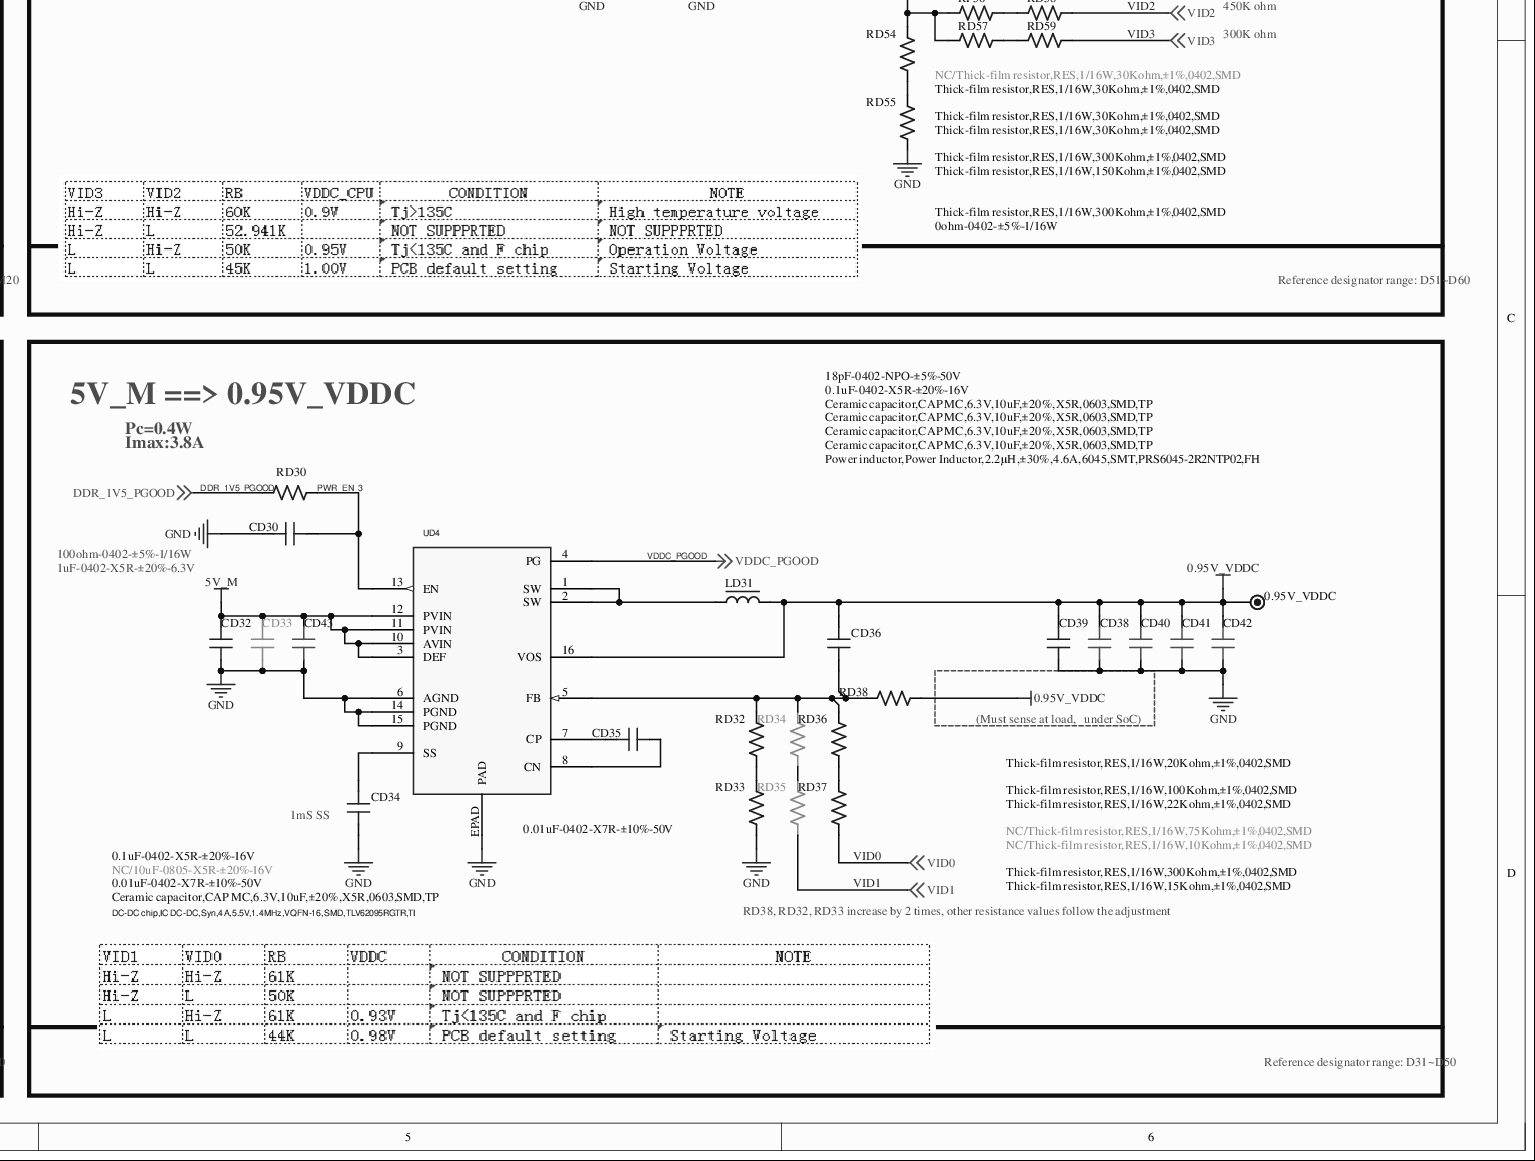
[diagram p0: MISC86290-6.SchDoc, bottom right]
# Altium project MISC86290.PrjPcb (part 5 of 13)

## Sheet MISC86290-6.SchDoc (continued)

### Parts
0.95V_VDDC  TEST  [TP]  (value not drawn)
1V5_DDR  TEST  [TP]  (value not drawn)
3V3_M  TEST  [TP]  (value not drawn)
3V3_STB  TEST  [TP]  (value not drawn)
3V3_Tun  TEST  [TP]  (value not drawn)
5V_M  TEST  [TP]  (value not drawn)
C58  NC/Ceramic capacitor,CAP MC,16V,0.1uF,±20%,X5R,0402,SMD,TP  [C0402]
CD1  NC/10uF-1206-X5R-±10%-16V  [C1206]
CD2  NC/1uF-0402-X5R-±20%-16V  [C0402]
CD3  10uF-0805-X5R-±20%-16V  [C0805]
CD4  NC/0.1uF-0402-X7R-±10%-16V  [C0402]
CD5  0.1uF-0402-X5R-±20%-16V  [C0402]
CD6  NC/8pF-0402-NPO-±5%-50V  [C0402]
CD7  NC/0.1uF-0402-X5R-±20%-16V  [C0402]
CD8  NC/Ceramic capacitor,CAP MC,6.3V,10uF,±20%,X5R,0603,SMD,TP  [C0603]
CD9  NC/Ceramic capacitor,CAP MC,6.3V,10uF,±20%,X5R,0603,SMD,TP  [C0603]
CD10  Ceramic capacitor,CAP MC,6.3V,10uF,±20%,X5R,0603,SMD,TP  [C0603]
CD11  10uF-0805-X5R-±20%-16V  [C0805]
CD12  NC/0.1uF-0402-X5R-±20%-16V  [C0402]
CD13  NC/10uF-1206-X5R-±10%-16V  [C1206]
CD14  0.1uF-0402-X5R-±20%-16V  [C0402]
CD15  NC/8pF-0402-NPO-±5%-50V  [C0402]
CD16  NC/0.1uF-0402-X5R-±20%-16V  [C0402]
CD17  Ceramic capacitor,CAP MC,6.3V,10uF,±20%,X5R,0603,SMD,TP  [C0603]
CD18  Ceramic capacitor,CAP MC,6.3V,10uF,±20%,X5R,0603,SMD,TP  [C0603]
CD19  Ceramic capacitor,CAP MC,6.3V,10uF,±20%,X5R,0603,SMD,TP  [C0603]
CD21  Ceramic capacitor,CAP MC,6.3V,10uF,±20%,X5R,0603,SMD,TP  [C0603]
CD22  0.1uF-0402-X7R-±10%-16V  [C0402]
CD23  Ceramic capacitor,CAP MC,50V,18pF,±5%,NPO,0402,SMD,TP  [C0402]
CD25  Ceramic capacitor,CAP MC,6.3V,10uF,±20%,X5R,0603,SMD,TP  [C0603]
CD26  Ceramic capacitor,CAP MC,6.3V,10uF,±20%,X5R,0603,SMD,TP  [C0603]
CD27  Ceramic capacitor,CAP MC,6.3V,22uF,±20%,X5R,0603,SMD,TP  [C0603]
CD29  0.1uF-0402-X7R-±10%-16V  [C0402]
CD30  1uF-0402-X5R-±20%-6.3V  [C0402]
CD32  0.1uF-0402-X5R-±20%-16V  [C0402]
CD33  NC/10uF-0805-X5R-±20%-16V  [C0805]
CD34  0.01uF-0402-X7R-±10%-50V  [C0402]
CD35  0.01uF-0402-X7R-±10%-50V  [C0402]
CD36  18pF-0402-NPO-±5%-50V  [C0402]
CD38  Ceramic capacitor,CAP MC,6.3V,10uF,±20%,X5R,0603,SMD,TP  [C0603]
CD39  0.1uF-0402-X5R-±20%-16V  [C0402]
CD40  Ceramic capacitor,CAP MC,6.3V,10uF,±20%,X5R,0603,SMD,TP  [C0603]
CD41  Ceramic capacitor,CAP MC,6.3V,10uF,±20%,X5R,0603,SMD,TP  [C0603]
CD42  Ceramic capacitor,CAP MC,6.3V,10uF,±20%,X5R,0603,SMD,TP  [C0603]
CD43  Ceramic capacitor,CAP MC,6.3V,10uF,±20%,X5R,0603,SMD,TP  [C0603]
CD51  Ceramic capacitor,CAP MC,6.3V,10uF,±20%,X5R,0603,SMD,TP  [C0603]
CD52  1uF-0402-X5R-±20%-6.3V  [C0402]
CD53  Ceramic capacitor,CAP MC,50V,18pF,±5%,NPO,0402,SMD,TP  [C0402]
CD54  Ceramic capacitor,CAP MC,6.3V,10uF,±20%,X5R,0603,SMD,TP  [C0603]
CD55  Ceramic capacitor,CAP MC,6.3V,10uF,±20%,X5R,0603,SMD,TP  [C0603]
CD56  Ceramic capacitor,CAP MC,6.3V,22uF,±20%,X5R,0603,SMD,TP  [C0603]
CG1  NC/1uF-0402-X5R-±20%-6.3V  [C0402]
CG11  NC/1uF-0402-X5R-±20%-6.3V  [C0402]
CG30  NC/1uF-0402-X5R-±20%-6.3V  [C0402]
CL1  0.1uF-0402-X5R-±20%-16V  [C0402]
CL2  Ceramic capacitor,CAP MC,6.3V,10uF,±20%,X5R,0603,SMD,TP  [C0603]
CL3  NC/0.1uF-0402-X5R-±20%-16V  [C0402]
CL13  Ceramic capacitor,CAP MC,6.3V,10uF,±20%,X5R,0603,SMD,TP  [C0603]
CL25  NC/0.1uF-0402-X5R-±20%-16V  [C0402]
CL55  0.1uF-0402-X5R-±20%-16V  [C0402]
CM1  1uF-0402-X5R-±20%-6.3V  [C0402]
CM2  0.022uF-0402-X7R-±10%-16V  [C0402]
CM3  22uF-0603-X5R-±20%-6.3V  [C0603]
CM4  0.022uF-0402-X7R-±10%-16V  [C0402]
CM15  NC/0.1uF-0402-X5R-±20%-16V  [C0402]
CM16  0.022uF-0402-X7R-±10%-16V  [C0402]
CM17  NC/10uF-0805-X5R-±20%-16V  [C0805]
CM18  NC/10uF-0805-X5R-±20%-16V  [C0805]
CNP2  Connector socket,connect jack,2×8Pin,D2.0,D,SNAP,L=2.6mm,DIP,CNJST  [SIP2*8/2.0D-5]
CP1  10uF-0805-X5R-±20%-16V  [C0805]
CP2  NC/0.1uF-0402-X5R-±20%-16V  [C0402]
DG1  NC/SFI0402-240E-2R5PP-LF  [DIODE-S0402]
DG11  NC/SFI0402-240E-2R5PP-LF  [DIODE-S0402]
DM11  NC/Switching diode,DIO SW S,150mA,75V,SOD-323,SMD,1N4148WS,BLUE ROCKET  [DIODE-S-12]
ED1  Aluminium electrolytic capacitor,CAP AL,10V,470uF,±20%,PKZH,P,2.5mm,6.3×11,DIP,TP,Koshin  [EC(6.3*11)-V-2.5]
EP1  Aluminium electrolytic capacitor,CAP AL,16V,220uF,±20%,LD,KF,P,2.5mm,6.3×11,DIP,TP,CapXon  [EC(6.3*11)-V-2.5]
LD1  NC/Power inductor,Power Inductor,4.7uH,±20%,3.3A,DR6.0×4.5,SMD,SWPA6045S4R7MT,Sunlord  [L(6.0*4.5)-S]
LD2  Power inductor,Power Inductor,4.7uH,±20%,2.8A,0.32×1P,DR5.8×4.5,SMD,PIO54-4R7MTP02,FH  [L(5.8*4.5)-S]
LD3  NC/Power inductor,Power Inductor,4.7uH,±20%,3.8A,DR6.0×4.5,SMD,MPIT6045-4R7M-LF,Microgate  [L(6.0*4.5)-S]
LD4  Power inductor,Power Inductor,4.7uH,±20%,3.3A,DR6.0×4.5,SMD,PRS6045-4R7MTP02,FH  [L(6.0*4.5)-S]
LD21  Power inductor,Power Inductor,2.2uH,±20%,2A,0.28×1P,DR4.5×3.2,SMD,PIO43-2R2MTP02,FH  [L(4.5*3.5)-S]
LD31  Power inductor,Power Inductor,2.2μH,±30%,4.6A,6045,SMT,PRS6045-2R2NTP02,FH  [L(6.0*4.5)-S]
LD51  Power inductor,Power Inductor,2.2uH,±20%,2A,0.28×1P,DR4.5×3.2,SMD,PIO43-2R2MTP02,FH  [L(4.5*3.5)-S]
MOD_1V2  TEST  [TP]
QG1  NC/General-purpose transistor,Dynatron,NPN,0.2A,40V,60-300,SOT-23,KMBT3904,KEXIN  [SOT-23]
QG2  NC/General-purpose transistor,Dynatron,NPN,0.2A,40V,60-300,SOT-23,KMBT3904,KEXIN  [SOT-23]
QG11  NC/General-purpose transistor,Dynatron,NPN,0.2A,40V,60-300,SOT-23,KMBT3904,KEXIN  [SOT-23]
QG12  NC/General-purpose transistor,Dynatron,NPN,0.2A,40V,60-300,SOT-23,KMBT3904,KEXIN  [SOT-23]
QG30  NC/General-purpose transistor,Dynatron,NPN,0.2A,40V,60-300,SOT-23,KMBT3904,KEXIN  [SOT-23]
QG31  NC/General-purpose transistor,Dynatron,NPN,0.2A,40V,60-300,SOT-23,KMBT3904,KEXIN  [SOT-23]
QM1  MOSFET,PMOS,-4.2A,-30V,0.052ohm@ID=-4.2A@VGS=-10V,SOT23-3,AO3401,BLUE ROCKET  [SOT-23-1]
QM2  MOSFET,PMOS,-5.7A,-30V,0.07ohm@ID=-4.4A@VGS=-4.5V,SOP-8,KO4459,KEXIN  [SO-8]
QM4  General-purpose transistor,Dynatron,NPN,0.2A,40V,60-300,SOT-23,KMBT3904,KEXIN  [SOT-23]
QM11  General-purpose transistor,Dynatron,NPN,0.2A,40V,60-300,SOT-23,KMBT3904,KEXIN  [SOT-23]
RD1  100ohm-0402-±5%-1/16W  [R0402]
RD2  NC/1Mohm-0402-±5%-1/16W  [R0402]
RD3  0ohm-0402-±5%-1/16W  [R0402]
RD4  0ohm-0402-±5%-1/16W  [R0402]
RD5  Thick-film resistor,RES,1/16W,59Kohm,±1%,0402,SMD  [R0402]
RD6  Thick-film resistor,RES,1/16W,10Kohm,±1%,0402,SMD  [R0402]
RD11  10Kohm-0402-±5%-1/16W  [R0402]
RD12  10Kohm-0402-±5%-1/16W  [R0402]
RD13  0ohm-0402-±5%-1/16W  [R0402]
RD14  0ohm-0402-±5%-1/16W  [R0402]
RD15  33Kohm-0402-±1%-1/16W  [R0402]
RD16  10Kohm-0402-±1%-1/16W  [R0402]
RD21  100Kohm-0402-±5%-1/16W  [R0402]
RD22  Thick-film resistor,RES,1/16W,15Kohm,±1%,0402,SMD  [R0402]
RD23  Thick-film resistor,RES,1/16W,10Kohm,±1%,0402,SMD  [R0402]
RD24  10Kohm-0402-±5%-1/16W  [R0402]
RD30  100ohm-0402-±5%-1/16W  [R0402]
RD32  Thick-film resistor,RES,1/16W,100Kohm,±1%,0402,SMD  [R0402]
RD33  Thick-film resistor,RES,1/16W,22Kohm,±1%,0402,SMD  [R0402]
RD34  NC/Thick-film resistor,RES,1/16W,75Kohm,±1%,0402,SMD  [R0402]
RD35  NC/Thick-film resistor,RES,1/16W,10Kohm,±1%,0402,SMD  [R0402]
RD36  Thick-film resistor,RES,1/16W,300Kohm,±1%,0402,SMD  [R0402]
RD37  Thick-film resistor,RES,1/16W,15Kohm,±1%,0402,SMD  [R0402]
RD38  Thick-film resistor,RES,1/16W,20Kohm,±1%,0402,SMD  [R0402]
RD51  NC/0ohm-0402-±5%-1/16W  [R0402]
RD52  10Kohm-0402-±5%-1/16W  [R0402]
RD53  NC/Thick-film resistor,RES,1/16W,30Kohm,±1%,0402,SMD  [R0402]
RD54  Thick-film resistor,RES,1/16W,30Kohm,±1%,0402,SMD  [R0402]
RD55  Thick-film resistor,RES,1/16W,30Kohm,±1%,0402,SMD  [R0402]
RD57  Thick-film resistor,RES,1/16W,300Kohm,±1%,0402,SMD  [R0402]
RD58  Thick-film resistor,RES,1/16W,150Kohm,±1%,0402,SMD  [R0402]
RD59  0ohm-0402-±5%-1/16W  [R0402]
RD60  Thick-film resistor,RES,1/16W,30Kohm,±1%,0402,SMD  [R0402]
RF56  Thick-film resistor,RES,1/16W,300Kohm,±1%,0402,SMD  [R0402]
RG1  NC/1Kohm-0402-±5%-1/16W  [R0402]
RG2  NC/4K7ohm-0402-±5%-1/16W  [R0402]
RG3  NC/33ohm-0402-±5%-1/16W  [R0402]
RG4  4K7ohm-0402-±5%-1/16W  [R0402]
RG5  100ohm-0402-±5%-1/16W  [R0402]
RG6  NC/10Kohm-0402-±5%-1/16W  [R0402]
RG7  NC/1Kohm-0402-±5%-1/16W  [R0402]
RG8  NC/10Kohm-0402-±5%-1/16W  [R0402]
RG11  NC/10Kohm-0402-±5%-1/16W  [R0402]
RG12  NC/1Kohm-0402-±5%-1/16W  [R0402]
RG13  NC/33ohm-0402-±5%-1/16W  [R0402]
RG14  4K7ohm-0402-±5%-1/16W  [R0402]
RG15  100ohm-0402-±5%-1/16W  [R0402]
RG16  NC/10Kohm-0402-±5%-1/16W  [R0402]
RG17  NC/1Kohm-0402-±5%-1/16W  [R0402]
RG18  NC/10Kohm-0402-±5%-1/16W  [R0402]
RG30  NC/4K7ohm-0402-±5%-1/16W  [R0402]
RG31  4K7ohm-0402-±5%-1/16W  [R0402]
RG32  NC/100ohm-0402-±5%-1/16W  [R0402]
RG33  100ohm-0402-±5%-1/16W  [R0402]
RG34  NC/10Kohm-0402-±5%-1/16W  [R0402]
RG35  0ohm-0402-±5%-1/16W  [R0402]
RG36  NC/10Kohm-0402-±5%-1/16W  [R0402]
RG37  NC/1Kohm-0402-±5%-1/16W  [R0402]
RG38  NC/1Kohm-0402-±5%-1/16W  [R0402]
RG39  NC/33ohm-0402-±5%-1/16W  [R0402]
RG40  NC/2K2ohm-0402-±5%-1/16W  [R0402]
RM1  15Kohm-0402-±1%-1/16W  [R0402]
RM2  4K7ohm-0402-±5%-1/16W  [R0402]
RM3  47Kohm-0402-±5%-1/16W  [R0402]
RM4  1Kohm-0402-±5%-1/16W  [R0402]
RM11  4K7ohm-0402-±5%-1/16W  [R0402]
RM12  10Kohm-0402-±5%-1/16W  [R0402]
RM13  4K7ohm-0402-±5%-1/16W  [R0402]
RM14  47Kohm-0402-±5%-1/16W  [R0402]
RM15  NC/4K7ohm-0402-±5%-1/16W  [R0402]
RP1  4K7ohm-0402-±5%-1/16W  [R0402]
RP5  NC/4K7ohm-0402-±5%-1/16W  [R0402]
RP8  100ohm-0402-±5%-1/16W  [R0402]
UD1  DC-DC chip,IC DCDC,Syn,4A,17V,500KHz,SOT23-6,SMD,TPS564201,TI  [SOP6/0.95]
UD2  DC-DC chip,IC DCDC,Syn,3A,17V,580KHz,TSOT23-6,SMD,TPS563201DDCR,TI  [SOP6/0.95]
UD3  DC-DC chip,IC DCDC,Syn,2A,5.5V,1.5MHz,SOT23-6,SMD,TLV62569PDDCR,TI  [SOT-23-6]
UD4  DC-DC chip,IC DC-DC,Syn,4A,5.5V,1.4MHz,VQFN-16,SMD,TLV62095RGTR,TI  [QFN16/0.5-4]
UD5  DC-DC chip,IC DCDC,Syn,2A,5.5V,1.5MHz,SOT23-6,SMD,TLV62569PDDCR,TI  [SOT-23-6]
UL1  LC1117CLTR33  [SOT-223]
UL2  LDO chip,IC LDO,1A,1.2V,15V,SOT-223,SMD,LC1117CLTR12,Leadchip  [SOT-223]
VCC_Panel  TEST  [TP]  (value not drawn)

### Blocks framed on the sheet
Power interface: CNP2 CP1 CP2 EP1 RP1 RP5 RP8
12V=>5V_M: 5V_M CD1-CD10 ED1 LD1 LD4 RD1-RD6 UD1
12V=>3V3_STB: 3V3_STB CD11-CD19 CD29 LD2 LD3 RD11-RD16 UD2
3V3_STB =>1V5_DDR: 1V5_DDR C58 CD21-CD23 CD25-CD27 LD21 RD21-RD24 UD3
5V_M ==> 0.95V_VDDCPU: CD51-CD56 LD51 RD51-RD55 RD57-RD60 RF56 UD5
PANEL VCC: CM15-CM18 DM11 QM2 QM11 RM11-RM15 VCC_Panel
3V3_STB=>3V3_M: 3V3_M CM1-CM4 QM1 QM4 RM1-RM4
BL_ON: CG1 DG1 QG1 QG2 RG1-RG8
5V_M ==> 0.95V_VDDC: 0.95V_VDDC CD30 CD32-CD36 CD38-CD43 LD31 RD30 RD32-RD38 UD4
PWM/ADJ: CG11 DG11 QG11 QG12 RG11-RG18
ADIM: CG30 QG30 QG31 RG30-RG40

### Nets
0.95V_VDDC: 0.95V_VDDC.1 CD36.2 CD38.2 CD39.2 CD40.2 CD41.2 CD42.2 LD31.2 RD38.2 UD4.16(VOS)
0.95V_VDDCPU: CD53.2 CD54.2 CD55.2 CD56.2 LD51.2 RD53.2 RD60.1
1V5_DDR: 1V5_DDR.1 C58.2 CD23.2 CD25.2 CD26.2 CD27.2 LD21.2 RD22.2
3V3_M: 3V3_M.1 CL55.2 CM2.2 CM3.2 QM1.D RD24.2 RG6.2 RG16.2 RP5.2 UL2.3(VI)
3V3_STB: 3V3_STB.1 CD15.2 CD16.2 CD17.2 CD18.2 CD19.2 CD21.2 CM4.2 LD2.1 LD3.2 QM1.S RD15.1 RD21.2 RG7.2 RG17.2 RG30.2 RG38.2 RM2.1 RP1.2 UD3.4(VIN)
3V3_Tun: 3V3_Tun.1 CL2.2 CL3.1 UL1.2(VO) UL1.4(VO)
5V_M: 5V_M.1 CD7.2 CD8.2 CD9.2 CD10.2 CD32.2 CD33.1 CD43.2 CD51.2 CL1.1 ED1.1 LD1.2 LD4.2 RD5.1 RD52.2 RG1.2 RG12.2 RG37.2 UD4.3(DEF) UD4.10(AVIN) UD4.11(PVIN) UD4.12(PVIN) UD5.4(VIN) UL1.3(VI)
12V: CD1.2 CD2.2 CD3.1 CD11.1 CD12.2 CD13.2 CM15.2 CNP2.5 CNP2.6 CNP2.7 CNP2.8 CP1.2 CP2.2 EP1.1 QM2.1(S) QM2.2(S) QM2.3(S) RD11.1 RM13.1 UD1.3(IN) UD2.3(IN)
AMP_VCC: CNP2.1 CNP2.2
GND: C58.1 CD1.1 CD2.1 CD3.2 CD4.2 CD6.1 CD7.1 CD8.1 CD9.1 CD10.1 CD11.2 CD12.1 CD13.1 CD16.1 CD17.1 CD18.1 CD19.1 CD21.1 CD22.2 CD25.1 CD26.1 CD27.1 CD29.2 CD30.1 CD32.1 CD33.2 CD34.1 CD38.1 CD39.1 CD40.1 CD41.1 CD42.1 CD43.1 CD51.1 CD52.2 CD54.1 CD55.1 CD56.1 CG1.1 CG11.1 CG30.1 CL1.2 CL2.1 CL3.2 CL13.1 CL25.1 CL55.1 CM1.1 CM3.1 CM17.2 CM18.2 CNP2.3 CNP2.4 CNP2.9 CNP2.10 CNP2.11 CNP2.12 CP1.1 CP2.1 DG1.A DG11.A ED1.2 EP1.2 QG1.E QG2.E QG11.E QG12.E QG30.E QG31.E QM4.E QM11.E RD2.1 RD6.1 RD12.1 RD16.1 RD23.1 RD33.1 RD55.1 RG4.1 RG14.1 RG31.1 RG40.1 RM12.1 RM15.2 UD1.1(GND) UD2.1(GND) UD3.2(GND) UD4.6(AGND) UD4.14(PGND) UD4.15(PGND) UD4.EPAD(PAD) UD5.2(GND) UL1.1(ADJ) UL2.1(ADJ)
MOD_1V2: CL13.2 CL25.2 MOD_1V2.1 UL2.2(VO) UL2.4(VO)
VCC_Panel: CM16.2 CM17.1 CM18.1 QM2.5(D) QM2.6(D) QM2.7(D) QM2.8(D) RM15.1 VCC_Panel.1
BL_ADIM: CG30.2 CNP2.14 RG35.1 RG39.2 RG40.2
BL_ON: CG1.2 CNP2.15 RG3.1 RG4.2 RG5.1
DDR_1V5_PGOOD: RD24.1 RD30.1 RD51.2 UD3.5(PG) ; off-sheet DDR_1V5_PGOOD
PS_ON: CNP2.13 RP5.1 RP8.1
PWM/ADJ: CG11.2 CNP2.16 RG13.2 RG14.2 RG15.1
PWR_EN_3: CD30.2 RD30.2 UD4.13(EN)
SOC_BL_ADIM: RG33.1 ; off-sheet SOC_BL_ADIM
SOC_BL_ON: DG1.K RG2.2 RG5.2 RG6.1 ; off-sheet SOC_BL_ON
SOC_BL_PDIM: DG11.K RG11.2 RG15.2 RG16.1 ; off-sheet SOC_BL_PDIM
SOC_BOOSTER: RG32.1 ; off-sheet SOC_BOOSTER
SOC_PANEL_ON: RM11.1 RM12.2 ; off-sheet SOC_PANEL_ON
SOC_PS_ON: RD1.1 RM1.1 RP1.1 RP8.2 ; off-sheet SOC_PS_ON
VDDC_PGOOD: UD4.4(PG) ; off-sheet VDDC_PGOOD
VDDCPU_PGOOD: UD5.5(PG) ; off-sheet VDDCPU_PGOOD
VID0: RD37.1 ; off-sheet VID0
VID1: RD35.1 ; off-sheet VID1
VID2: RD58.1 ; off-sheet VID2
VID3: RD59.1 ; off-sheet VID3
NetCD4_1: CD4.1 RD1.2 RD2.2 UD1.5(EN)
NetCD5_1: CD5.1 RD3.2
NetCD5_2: CD5.2 LD1.1 LD4.1 UD1.2(SW)
NetCD6_2: CD6.2 RD4.1 UD1.4(FB)
NetCD14_1: CD14.1 LD2.2 LD3.1 UD2.2(SW)
NetCD14_2: CD14.2 RD13.2
NetCD15_1: CD15.1 RD14.2 RD15.2 RD16.2
NetCD22_1: CD22.1 RD21.1 UD3.1(EN)
NetCD23_1: CD23.1 RD22.1 RD23.2 UD3.6(FB)
NetCD29_1: CD29.1 RD11.2 RD12.2 UD2.5(EN)
NetCD34_2: CD34.2 UD4.9(SS)
NetCD35_1: CD35.1 UD4.8(CN)
NetCD35_2: CD35.2 UD4.7(CP)
NetCD36_1: CD36.1 RD32.1 RD34.1 RD36.1 RD38.1 UD4.5(FB)
NetCD52_1: CD52.1 RD51.1 RD52.1 UD5.1(EN)
NetCD53_1: CD53.1 RD53.1 RD54.2 RD57.2 RD60.2 RF56.2 UD5.6(FB)
NetCM1_2: CM1.2 QM4.B RM1.2
NetCM2_1: CM2.1 RM4.2
NetCM4_1: CM4.1 QM1.G RM3.2 RM4.1
NetCM15_1: CM15.1 CM16.1 DM11.K QM2.4(G) RM14.2
NetDM11_A: DM11.A QM11.C RM13.2 RM14.1
NetLD21_1: LD21.1 UD3.3(SW)
NetLD31_1: LD31.1 UD4.1(SW) UD4.2(SW)
NetLD51_1: LD51.1 UD5.3(SW)
NetQG1_B: QG1.B RG8.1
NetQG1_C: QG1.C RG1.1 RG3.2
NetQG2_B: QG2.B RG2.1
NetQG2_C: QG2.C RG7.1 RG8.2
NetQG11_B: QG11.B RG18.1
NetQG11_C: QG11.C RG12.1 RG13.1
NetQG12_B: QG12.B RG11.1
NetQG12_C: QG12.C RG17.1 RG18.2
NetQG30_B: QG30.B RG34.1
NetQG30_C: QG30.C RG36.2 RG38.1
NetQG31_B: QG31.B RG36.1
NetQG31_C: QG31.C RG37.1 RG39.1
NetQM4_C: QM4.C RM2.2 RM3.1
NetQM11_B: QM11.B RM11.2
NetRD3_1: RD3.1 UD1.6(BS)
NetRD4_2: RD4.2 RD5.2 RD6.2
NetRD13_1: RD13.1 UD2.6(BS)
NetRD14_1: RD14.1 UD2.4(FB)
NetRD32_2: RD32.2 RD33.2
NetRD34_2: RD34.2 RD35.2
NetRD36_2: RD36.2 RD37.2
NetRD54_1: RD54.1 RD55.2
NetRD57_1: RD57.1 RD59.2
NetRD58_2: RD58.2 RF56.1
NetRG30_1: RG30.1 RG31.2 RG32.2 RG33.2 RG34.2 RG35.2

### Notes on the sheet
- Imax:3.6A
- Pc=0.44W
- Pc=0.88W
- Imax:2.4A
- STR
- Imax:1A
- Pc=0.15W
- All close to the power terminal
- Vout=0.6*(1+RD22/RD23)=1.5V
- Reference designator range: D21~D30
- TPS564201:  Vout=0.768*(1+RD9/RD7)=0.768*(1+59/10) = 5.24V
- Reference designator range: D1~D10
- TPS563201:  Vout=0.768*(1+RD15/RD16)=0.768*(1+33/10) = 3.3V
- Reference designator range: D11~D20
- H :Power on
- Pc=0.16W
- (near RP1) L :Power off
- Imax:1.5A
- Current:350mA
- PANEL_EN_IC
- L
- H
- Panel VCC
- ON
- OFF
- (near CM18) Place close to the panel interface
- Note:
- 1、Amplifier power is taken from AMP_VCC (12V/18V/24V); if the power board outputs only 12V, place RP7
- 2、This circuit requires the BackLight-External circuit
- (near RD58) Remote SOC feedback
- 450K ohm
- Revision: Power Interface-Single TV-B-V1.0
- Reference designator range: P1~P10
- 300K ohm
- Reference designator range: M11~M20
- Reference designator range: D51~D60
- Power on sequence: XTAL > 3V3_STB > Reset > 3V3_M > 1.5V_DDR > 1.1V_VDDC
- Reference designator range: M1~M10
- 5V_M=>3V3_Tun
- 3V3_M=>MOD_1V2
- Imax:0.25A
- Pc=0.425W
- Imax:0.1A
- Pc=0.2W
- Imax:3.8A
- Pc=0.4W
- Reference designator range: G1~G10
- (Must sense at load,   under SoC)
- (near CD34) 1mS SS
- RD38, RD32, RD33 increase by 2 times, other resistance values follow the adjustment
- Reference designator range: G30~G40
- Reference designator range: G11~G20
- Reference designator range: L1~L10
- Reference designator range: D31~D50

### Library data of the parts
C58 = 004.003.0000403-D: Ceramic capacitor,CAP MC,16V,0.1uF,±20%,X5R,0402,SMD,TP-D
CD1 CD13 = 10uF-1206-X5R-±10%-16V-D
CD2 CD5 CD7 CD32 CD39 CP2 = 0.1uF-0402-Y5V-+80%-20%-16V-D
CD3 CD11 CD33 CM17 CM18 CP1 = 10uF-0805-X5R-±20%-16V-D
CD4 CD12 CD14 CD16 CD22 CD29 CD30 CD52 CL1 CL3 CL25 CL55 = 0.1uF-0402-X5R-±20%-16V-D
CD6 = 10pF-0402-NPO-±5%-50V-D
CD8-CD10 CD17-CD19 CD21 CD25 CD26 CD38 CD40-CD43 CD51 CD54 CD55 CL2 CL13 = 004.003.0000383-D: Ceramic capacitor,CAP MC,6.3V,10uF,±20%,X5R,0603,SMD,TP-D
CD15 = 8pF-0402-NPO-±5%-50V-D
CD23 CD53 = 004.003.0000527-D: Ceramic capacitor,CAP MC,50V,18pF,±5%,NPO,0402,SMD,TP-D
CD27 CD56 = 004.003.0000671-D: Ceramic capacitor,CAP MC,6.3V,22uF,±20%,X5R,0603,SMD,TP-D
CD34 CM2 CM4 CM16 = 0.022uF-0402-X7R-±10%-16V-D
CD35 = 0.01uF-0402-X7R-±10%-50V-D
CD36 = 120pF-0402-NPO-±5%-50V-D
CG1 CG11 CG30 = 1uF-0402-X5R-±20%-6.3V-D
CM1 = 1000pF-0402-X7R-±10%-50V-D
CM3 = 22uF-0603-X5R-±20%-6.3V-D
CM15 = 0.1uF-0402-X7R-±10%-16V-D
CNP2 = 2×8PIN-2.0-D-H-G-带扣-J-DHMI: CN-keyed
DG1 DG11 = AVLC18S02003-D
DM11 = 1N4148WS-D
ED1 = 470uF-10V-±20%-6.3×11-105℃-黑底白字-编带-F=2.5-XF-DHAI: Electrolytic
EP1 = 004.003.0000158-DHAI: Aluminium electrolytic capacitor,CAP AL,16V,220uF,±20%,LD,KF,P,2.5mm,6.3×11,DIP,TP,CapXon-DHAI
LD1 LD3 LD4 = SWPA6045S4R7MT-D
LD2 = MGSD54-6R8M-LF-D
LD21 LD51 = SLN43T-6R8M-D
LD31 = 004.004.0000652-D: Power inductor,Power Inductor,2.2uH,±20%,4.60A,DR6.0×4.5,SMD,MPIT6045-2R2M-LF,Microgate-D
QG1 QG2 QG11 QG12 QG30 QG31 = LMBT3904LT1G-D-NPN: Q-NPN-#-#-#
QM1 = WPM3407C-3/TR-D
QM2 = AO4459-D
QM4 QM11 = KMBT3904-D
RD1 RD11 RD12 RG32 RG33 = 100Kohm-0402-±5%-1/16W-D
RD2 = 1Mohm-0402-±5%-1/16W-D
RD3 RD4 RD13 RD14 RD30 RD51 = 0ohm-0402-±5%-1/16W-D
RD5 = 30Kohm-0402-±5%-1/16W-D
RD6 = 3K3ohm-0402-±5%-1/16W-D
RD15 RD38 = 60K4ohm-0402-±1%-1/16W-D
RD16 = 10K5ohm-0402-±1%-1/16W-D
RD21 RD24 RD52 = 004.002.0000689-D: Thick-film resistor,RES,1/16W,4.7Kohm,±5%,0402,SMD-D
RD22 RD53 RD60 = 004.002.0000718-D: Thick-film resistor,RES,1/16W,6.2Kohm,±1%,0402,SMD-D
RD23 RD54 RD55 RD57 RD59 = 004.002.0000622-D: Thick-film resistor,RES,1/16W,20Kohm,±1%,0402,SMD-D
RD32 RD34 RD36 = 113Kohm-0402-±1%-1/16W-D
RD33 RD35 RD37 = 47Kohm-0402-±1%-1/16W-D
RD58 = 004.002.0000558-D: Thick-film resistor,RES,1/16W,0ohm,±5%,0402,SMD-D
RF56 = 004.002.0000757-D: Thick-film resistor,RES,1/16W,120Kohm,±1%,0402,SMD-D
RG1 RG7 RG12 RG17 RG37 RG38 = 1Kohm-0402-±5%-1/16W-D
RG2 RG30 RG31 RM1 RM2 RM11 RM13 RM15 RP5 = 4K7ohm-0402-±5%-1/16W-D
RG3 RG13 RG39 = 33ohm-0402-±5%-1/16W-D
RG4 RG5 RG14 RG15 RG35 RG40 RP8 = 2K2ohm-0402-±5%-1/16W-D
RG6 RG8 RG11 RG16 RG18 RG34 RG36 RM12 RP1 = 10Kohm-0402-±5%-1/16W-D
RM3 RM4 RM14 = 47Kohm-0402-±5%-1/16W-D
UD1 = MP1470GJ-Z-D
UD2 = MP1471AGJ-Z-D
UD3 UD5 = 004.010.0000967-D: DC-DC chip,IC DCDC,Syn,2A,5.5V,1.5MHz,SOT23-6,SMD,TLV62569PDDCR,TI-D
UD4 = 004.010.0000812: DC-DC chip,IC DC-DC,Syn,4A,5.5V,1.4MHz,VQFN-16,SMD,TLV62095RGTR,TI-D
UL1 = LC1117CLTR33-D
UL2 = LC1117CLTRAD-D